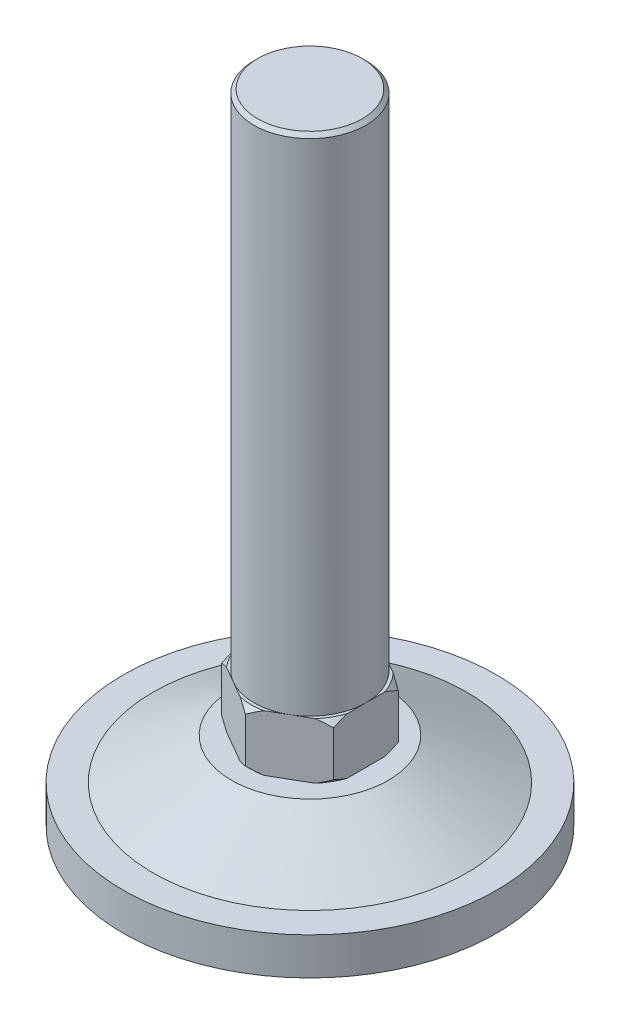
from build123d import *

# Parameters (mm, degrees)
BOSS_EXTRUDE1_DEPTH     = 15
CHAMFER1_SIZE           = 1
SKETCH4_R               = 79.861717746
SKETCH4_R_2             = 50
CUT_EXTRUDE1_DEPTH      = 182.991758055
CUT_EXTRUDE2_DEPTH      = 195.321897891
CUT_EXTRUDE2_DEPTH_BACK = 195.321897891
SKETCH5_W               = 151.709550381
SKETCH5_H               = 33.031628388


with BuildPart() as part:
    # Sketch1 → Revolve1 (revolve)
    with BuildSketch(Plane.XY, mode=Mode.PRIVATE) as revolve1_sk:
        Polygon((35, 0), (60, 0), (60, 9.5), (59.5, 10), (60, 10.5), (60, 20), (42, 20), (21, 31), (15, 31), (15, 181), (0, 181), (0, 15), (14, 15), align=None)
    revolve(revolve1_sk.sketch.rotate(Axis((0, 181, 0), (0, -1, 0)), 180), axis=Axis((0, 181, 0), (0, -1, 0)))

    # Sketch2 → Boss-Extrude1 (add)
    with BuildSketch(Plane(origin=(0, 31, 0), x_dir=(1, 0, 0), z_dir=(0, 1, 0))):
        Polygon((15, 8.660254038), (0, 17.320508076), (-15, 8.660254038), (-15, -8.660254038), (0, -17.320508076), (15, -8.660254038), align=None)
    extrude(amount=BOSS_EXTRUDE1_DEPTH)

    # Sketch3 → Cut-Revolve1 (revolve, cut)
    with BuildSketch(Plane(origin=(0, 0, 0), x_dir=(0, 0, -1), z_dir=(1, 0, 0))):
        Polygon((15.820508076, 31), (17.320508076, 32.5), (17.320508076, 31), align=None)
        Polygon((17.320508076, 44.5), (15.820508076, 46), (17.320508076, 46), align=None)
    revolve(axis=Axis((0, 181, 0), (0, 1, 0)), mode=Mode.SUBTRACT)

    # Chamfer1
    chamfer1_edges = [part.edges().sort_by_distance(p)[0] for p in [
        (15, 181, 0),
    ]]
    chamfer(chamfer1_edges, length=CHAMFER1_SIZE)

    # Sketch4 → Cut-Extrude1 (cut, through all)
    with BuildSketch(Plane(origin=(0, 20, 0), x_dir=(1, 0, 0), z_dir=(0, 1, 0))):
        Circle(SKETCH4_R)
        with Locations(Location((0, 0, 0), (0, 0, 180))):
            Circle(SKETCH4_R_2, mode=Mode.SUBTRACT)
    extrude(amount=-CUT_EXTRUDE1_DEPTH, mode=Mode.SUBTRACT)

    # Sketch5 → Cut-Extrude2 (cut, two sides: drawn at the far end of the back side and taken through both)
    with BuildSketch(Plane.XY.offset(-CUT_EXTRUDE2_DEPTH_BACK)):
        with Locations((18.277609901, -6.515814194)):
            Rectangle(SKETCH5_W, SKETCH5_H)
    extrude(amount=CUT_EXTRUDE2_DEPTH + CUT_EXTRUDE2_DEPTH_BACK, mode=Mode.SUBTRACT)


solid = part.part
